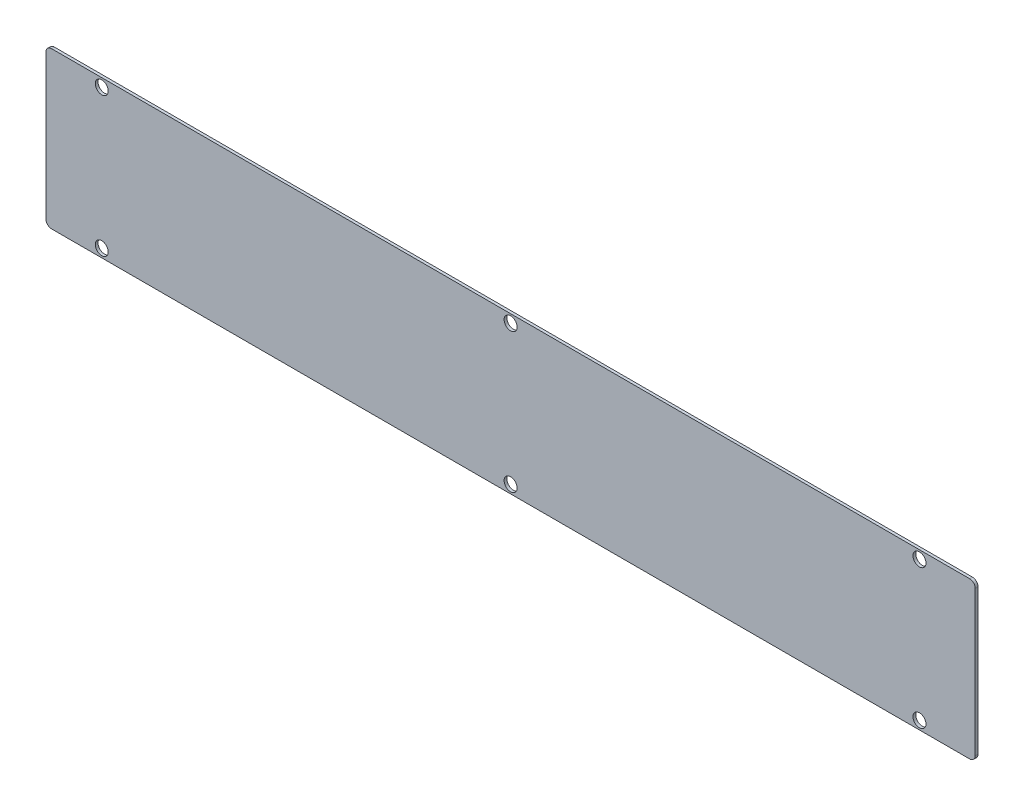
SolidWorks part; units mm, degrees
material "SUS 304"
ref_plane "前视基准面" through (0, 0, 0) normal (0, 0, 1) x (1, 0, 0)
ref_plane "上视基准面" through (0, 0, 0) normal (0, 1, 0) x (1, 0, 0)
ref_plane "右视基准面" through (0, 0, 0) normal (1, 0, 0) x (0, 0, -1)
sketch "草图1" plane through (0, 0, 0) normal (0, 0, 1) x (1, 0, 0)
  line L1 (-250, 42) -> (250, 42)
  line L2 (-250, 42) -> (-250, -42)
  line L3 (-250, -42) -> (250, -42)
  line L4 (250, 42) -> (250, -42)
  line L5 (-250, 42) -> (250, -42) construction
  line L6 (-250, -42) -> (250, 42) construction
  point P0 (0, 0)
  dimension "D1" = 500
  dimension "D2" = 84
extrude "凸台-拉伸1" add sketch "草图1" along normal blind 1.5
sketch "草图2" plane through (0, 0, 0) normal (0, 0, -1) x (-1, 0, 0)
  line L0 (-250, -42) -> (-250, 42) construction
  line L2 (-249, -42) -> (249, -42) construction
  line L4 (-250, 0) -> (-196.7114, 0) construction
  circle A0 centre (0, 37.5) radius 3.5
  circle A1 centre (220, 37.5) radius 3.5
  circle A2 centre (-220, -37.5) radius 3.5
  circle A3 centre (220, -37.5) radius 3.5
  circle A4 centre (0, -37.5) radius 3.5
  circle A5 centre (-220, 37.5) radius 3.5
  dimension "D2" = 220
  dimension "D3" = 4.5
  dimension "D4" = 7
  dimension "D5" = 7
  dimension "D6" = 7
  dimension "D7" = 220
  dimension "D11" = 0
extrude "切除-拉伸1" cut sketch "草图2" against normal through all
fillet "圆角1" radius 3 4 edges at (250, -42, 0.75) (250, 42, 0.75) (-250, -42, 0.75) (-250, 42, 0.75)
